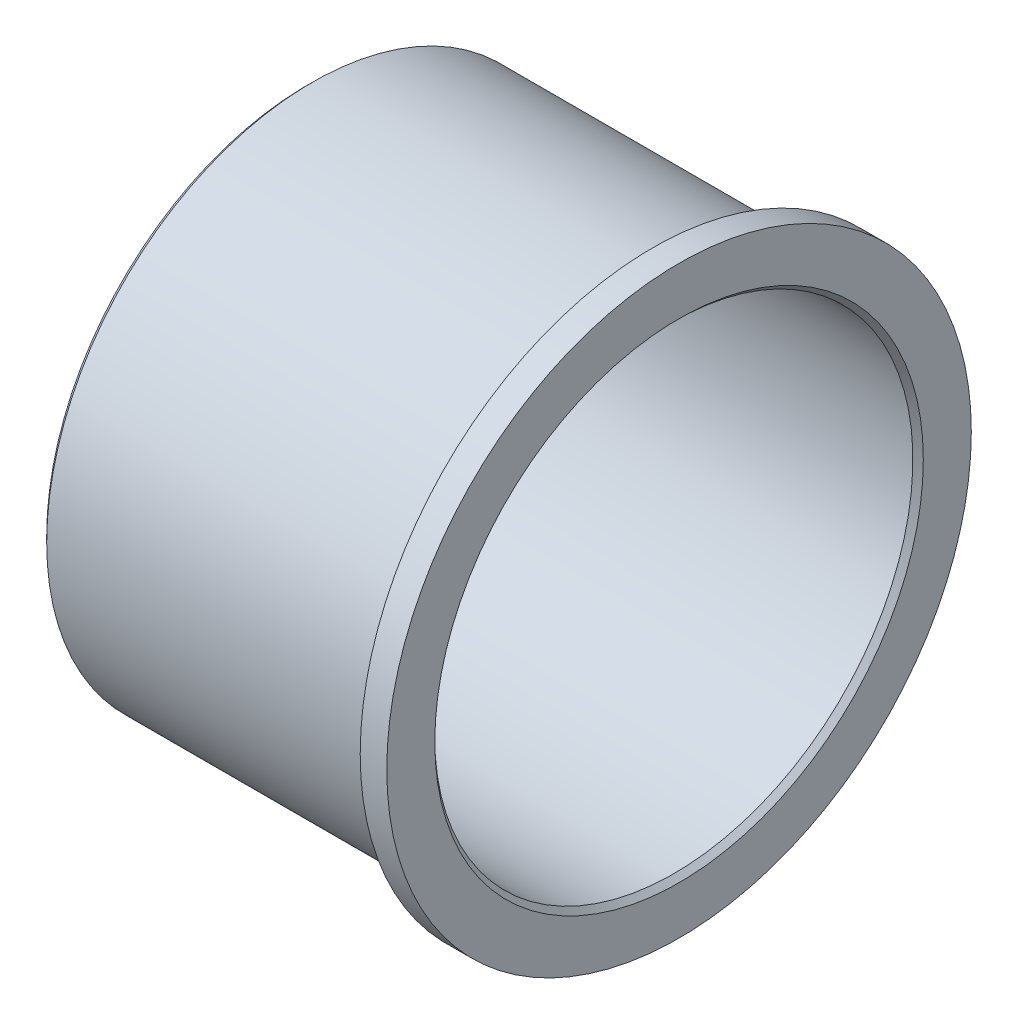
SolidWorks part; units mm, degrees
material "ZCuAL10Fe3#"
ref_plane "前视基准面" through (0, 0, 0) normal (0, 0, 1) x (1, 0, 0)
ref_plane "上视基准面" through (0, 0, 0) normal (0, 1, 0) x (1, 0, 0)
ref_plane "右视基准面" through (0, 0, 0) normal (1, 0, 0) x (0, 0, -1)
sketch "尺寸草图" plane through (0, 0, 0) normal (0, 0, 1) x (1, 0, 0)
  line L0 (-35, 0) -> (35, 0) construction
  line L1 (0, 0) -> (0, 45) construction
  line L2 (-35, 45.9657) -> (-34, 45)
  line L3 (-34, 45) -> (34, 45)
  line L4 (34, 45) -> (35, 45.9657)
  line L5 (35, 45.9657) -> (35, 55)
  line L6 (35, 55) -> (30, 55)
  line L7 (30, 55) -> (30, 49.8)
  line L8 (30, 49.8) -> (28, 49.8)
  line L9 (28, 49.8) -> (28, 50)
  line L10 (28, 50) -> (-34, 50)
  line L11 (-34, 50) -> (-35, 49)
  line L12 (-35, 49) -> (-35, 45.9657)
  dimension "D1" = 44
  dimension "内径d1" = 90
  dimension "倒角C1" = 1
  dimension "D2" = 0.2
  dimension "外径d2" = 100
  dimension "翻边外径d3" = 110
  dimension "宽度b1" = 70
  dimension "翻边宽度b2" = 5
  dimension "退刀槽宽度u" = 2
  dimension "倒角C2" = 1
  dimension "C2角度" = 45
revolve "旋转1" add sketch "尺寸草图" angle 360 about L0
